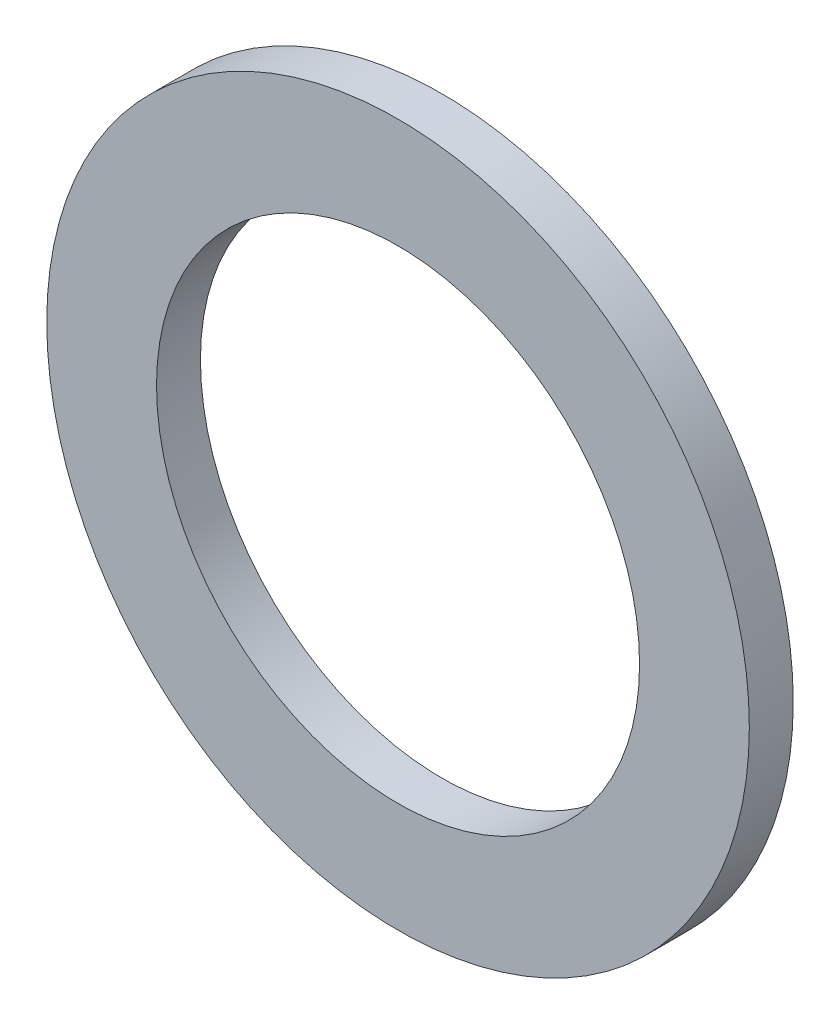
from build123d import *

# Parameters (mm, degrees)
SKETCH_1_R      = 8
SKETCH_1_R_2    = 5.5
EXTRUDE_1_DEPTH = 1


with BuildPart() as part:
    # 草图1 → 凸台-拉伸1 (new body)
    with BuildSketch(Plane.XY):
        Circle(SKETCH_1_R)
        Circle(SKETCH_1_R_2, mode=Mode.SUBTRACT)
    extrude(amount=EXTRUDE_1_DEPTH)


solid = part.part
